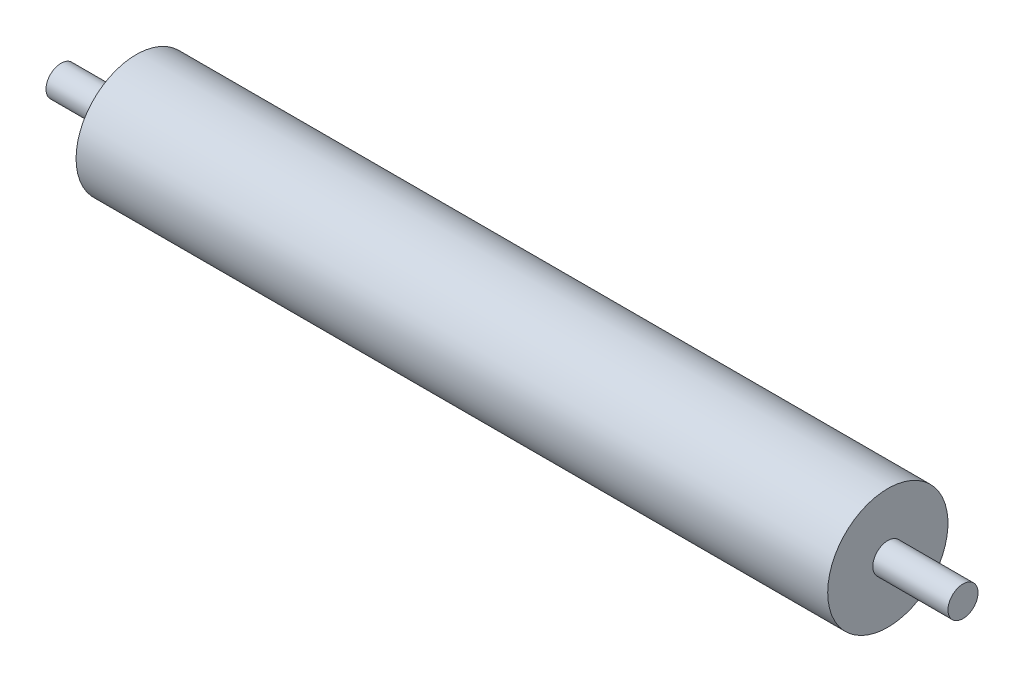
from build123d import *


with BuildPart() as part:
    # Sketch1 → Revolve1 (revolve)
    with BuildSketch(Plane.XY, mode=Mode.PRIVATE) as revolve1_sk:
        Polygon((-223.024643435, 190.413727793), (376.975356565, 190.413727793), (376.975356565, 200.413727793), (326.975356565, 200.413727793), (326.975356565, 230.413727793), (-173.024643435, 230.413727793), (-173.024643435, 200.413727793), (-223.024643435, 200.413727793), align=None)
    revolve(revolve1_sk.sketch.rotate(Axis((-223.024643435, 190.413727793, 0), (1, 0, 0)), 90), axis=Axis((-223.024643435, 190.413727793, 0), (1, 0, 0)))


solid = part.part
